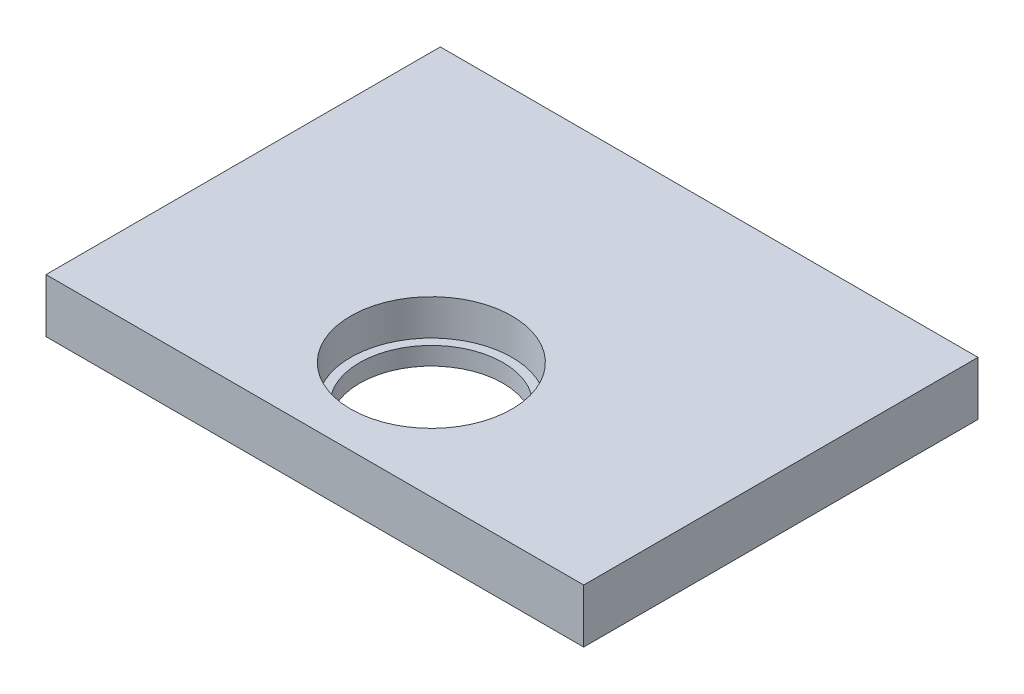
SolidWorks part; units mm, degrees
ref_plane "前视基准面" through (0, 0, 0) normal (0, 0, 1) x (1, 0, 0)
ref_plane "上视基准面" through (0, 0, 0) normal (0, 1, 0) x (1, 0, 0)
ref_plane "右视基准面" through (0, 0, 0) normal (1, 0, 0) x (0, 0, -1)
sketch "草图1" plane through (0, 0, 0) normal (0, 1, 0) x (1, 0, 0)
  line L1 (-150, -110) -> (150, -110)
  line L2 (-150, -110) -> (-150, 110)
  line L3 (-150, 110) -> (150, 110)
  line L4 (150, -110) -> (150, 110)
  line L5 (-150, -110) -> (150, 110) construction
  line L6 (-150, 110) -> (150, -110) construction
  point P0 (0, 0)
  dimension "D1" = 220
  dimension "D2" = 300
extrude "凸台-拉伸1" add sketch "草图1" along normal blind 30
sketch "草图2" plane through (0, 30, 0) normal (0, 1, 0) x (1, 0, 0)
  line L0 (150, -110) -> (150, 110) construction
  line L1 (150, 110) -> (-150, 110) construction
  circle A0 centre (0, -45) radius 45
  dimension "D1" = 90
  dimension "D2" = 150
  dimension "D3" = 155
extrude "切除-拉伸1" cut sketch "草图2" against normal blind 20
sketch "草图3" plane through (0, 30, 0) normal (0, 1, 0) x (1, 0, 0)
  line L0 (150, -110) -> (150, 110) construction
  line L1 (150, 110) -> (-150, 110) construction
  circle A0 centre (0, -45) radius 40
  dimension "D1" = 80
  dimension "D2" = 150
  dimension "D3" = 155
extrude "切除-拉伸2" cut sketch "草图3" against normal through all
